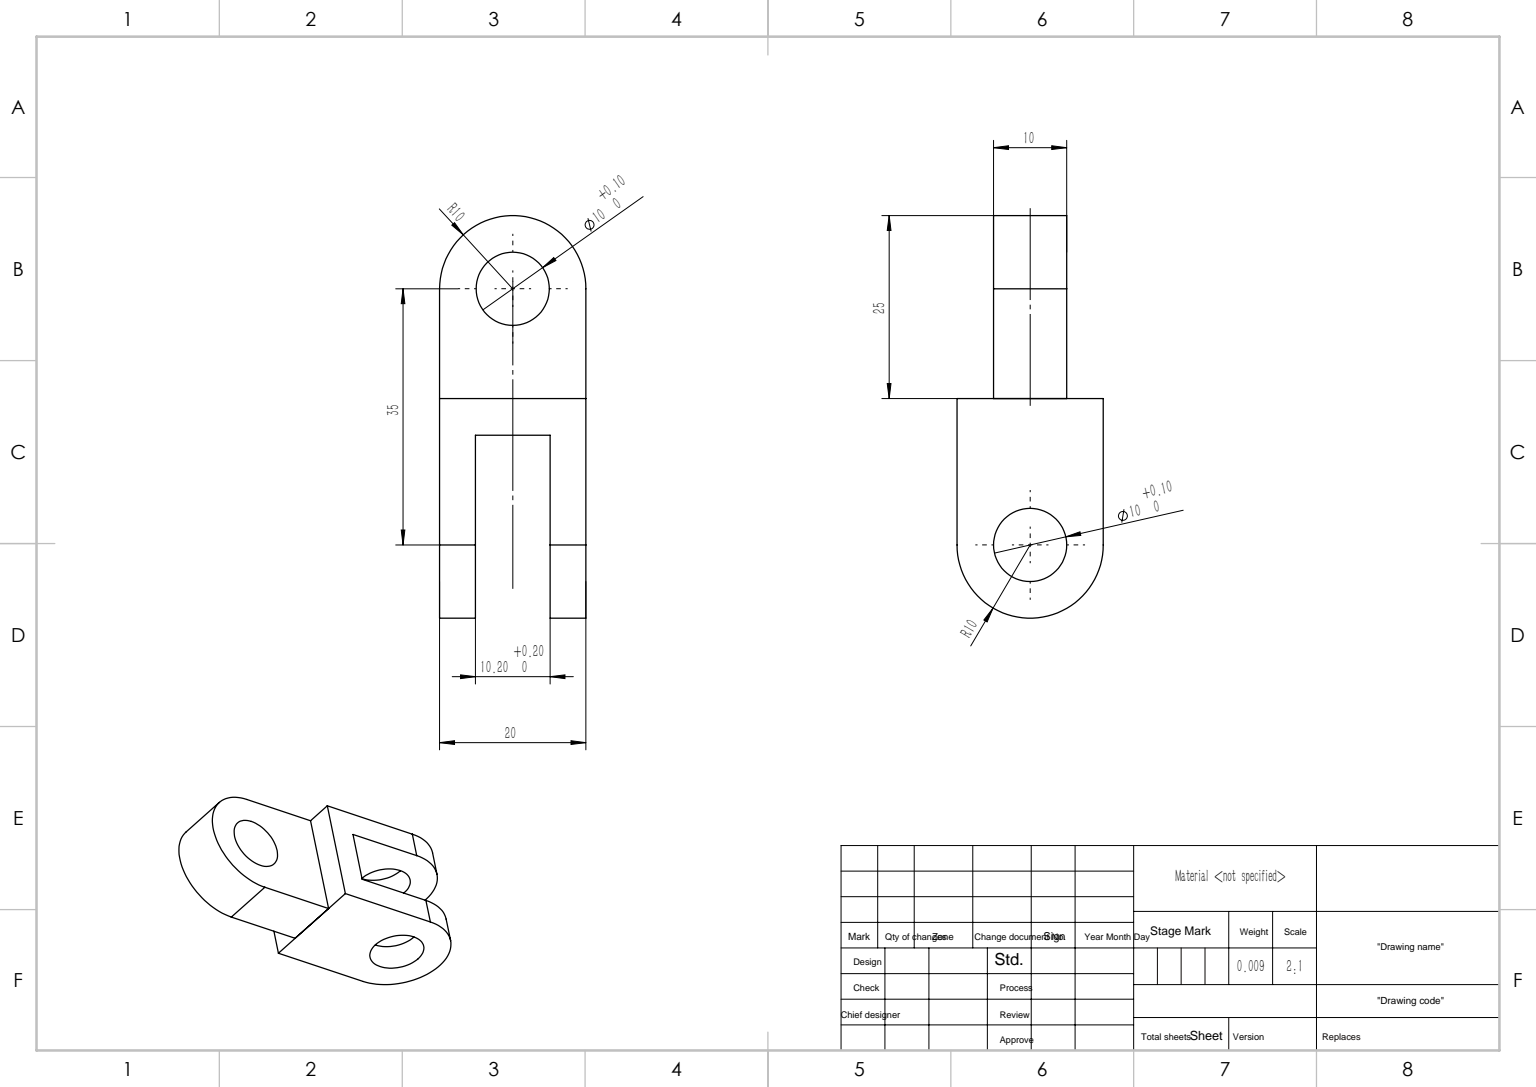
from build123d import *

# Parameters (mm, degrees)
SKETCH1_R           = 5
BOSS_EXTRUDE1_DEPTH = 10
SKETCH2_R           = 5
BOSS_EXTRUDE2_DEPTH = 20
SKETCH3_W           = 10.2
SKETCH3_H           = 29.458031572
CUT_EXTRUDE1_DEPTH  = 51.249378106


with BuildPart() as part:
    # Sketch1 → Boss-Extrude1 (new body)
    with BuildSketch(Plane.XY):
        with BuildLine():
            Line((-10, 0), (-10, -15))
            Line((-10, -15), (10, -15))
            Line((10, -15), (10, 0))
            ThreePointArc((10, 0), (0, 10), (-10, 0))
        make_face()
        Circle(SKETCH1_R, mode=Mode.SUBTRACT)
    extrude(amount=BOSS_EXTRUDE1_DEPTH)


with BuildPart() as body_2:
    # Sketch2 → Boss-Extrude2 (new body)
    with BuildSketch(Plane.ZY.offset(10)):
        with BuildLine():
            Line((15, -35), (15, -15))
            Line((15, -15), (-5, -15))
            Line((-5, -15), (-5, -35))
            ThreePointArc((-5, -35), (5, -45), (15, -35))
        make_face()
        with Locations(Location((5, -35, 0), (0, 0, 270))):
            Circle(SKETCH2_R, mode=Mode.SUBTRACT)
    extrude(amount=-BOSS_EXTRUDE2_DEPTH)

    # Sketch3 → Cut-Extrude1 (cut, through all)
    with BuildSketch(Plane(origin=(0, 0, -5), x_dir=(-1, 0, 0), z_dir=(0, 0, -1))):
        with Locations((0, -34.729015786)):
            Rectangle(SKETCH3_W, SKETCH3_H)
    extrude(amount=-CUT_EXTRUDE1_DEPTH, mode=Mode.SUBTRACT)


solid = Compound([part.part, body_2.part])
